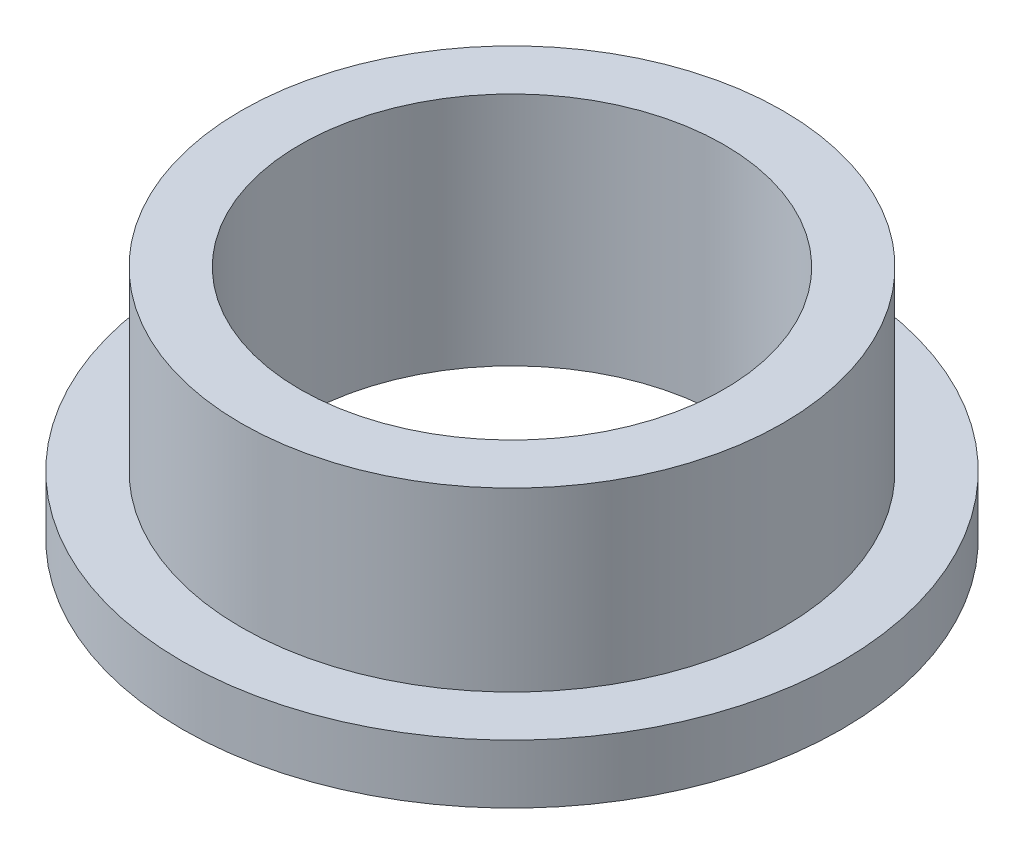
from build123d import *

# Parameters (mm, degrees)
SKETCH_1_R      = 28
SKETCH_1_R_2    = 18
EXTRUDE_1_DEPTH = 5
SKETCH_2_R      = 23
SKETCH_2_R_2    = 18
EXTRUDE_2_DEPTH = 15


with BuildPart() as part:
    # 草图1 → 凸台-拉伸1 (new body)
    with BuildSketch(Plane(origin=(0, 0, 0), x_dir=(1, 0, 0), z_dir=(0, 1, 0))):
        with Locations(Location((0, 0, 0), (0, 0, 270))):
            Circle(SKETCH_1_R)
        with Locations(Location((0, 0, 0), (0, 0, 270))):
            Circle(SKETCH_1_R_2, mode=Mode.SUBTRACT)
    extrude(amount=EXTRUDE_1_DEPTH)

    # 草图2 → 凸台-拉伸2 (add)
    with BuildSketch(Plane(origin=(0, 5, 0), x_dir=(1, 0, 0), z_dir=(0, 1, 0))):
        with Locations(Location((0, 0, 0), (0, 0, 270))):
            Circle(SKETCH_2_R)
        with Locations(Location((0, 0, 0), (0, 0, 270))):
            Circle(SKETCH_2_R_2, mode=Mode.SUBTRACT)
    extrude(amount=EXTRUDE_2_DEPTH)


solid = part.part
